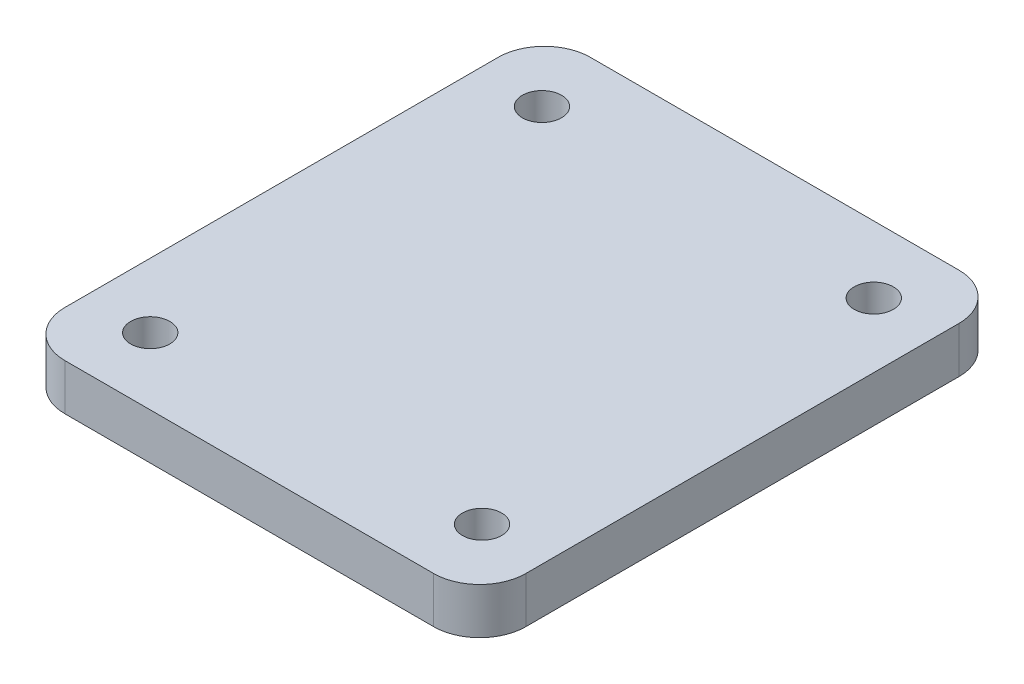
from build123d import *

# Parameters (mm, degrees)
BOSS_EXTRUDE1_DEPTH = 10
M10_TAPPED_HOLE1_D  = 8.5


with BuildPart() as part:
    # Sketch1 → Boss-Extrude1 (new body)
    with BuildSketch(Plane(origin=(0, 0, 0), x_dir=(1, 0, 0), z_dir=(0, 1, 0))):
        with BuildLine():
            Line((-40, -57), (40, -57))
            ThreePointArc((40, -57), (47.071067812, -54.071067812), (50, -47))
            Line((50, -47), (50, 47))
            ThreePointArc((50, 47), (47.071067812, 54.071067812), (40, 57))
            Line((40, 57), (-40, 57))
            ThreePointArc((-40, 57), (-47.071067812, 54.071067812), (-50, 47))
            Line((-50, 47), (-50, -47))
            ThreePointArc((-50, -47), (-47.071067812, -54.071067812), (-40, -57))
        make_face()
    extrude(amount=BOSS_EXTRUDE1_DEPTH)

    # M10 Tapped Hole1 (through all)
    with Locations(Plane(origin=(0, 10, 0), x_dir=(1, 0, 0), z_dir=(0, 1, 0))):
        with Locations((36, 42.5), (-36, -42.5), (-36, 42.5), (36, -42.5)):
            Hole(M10_TAPPED_HOLE1_D / 2)


solid = part.part
